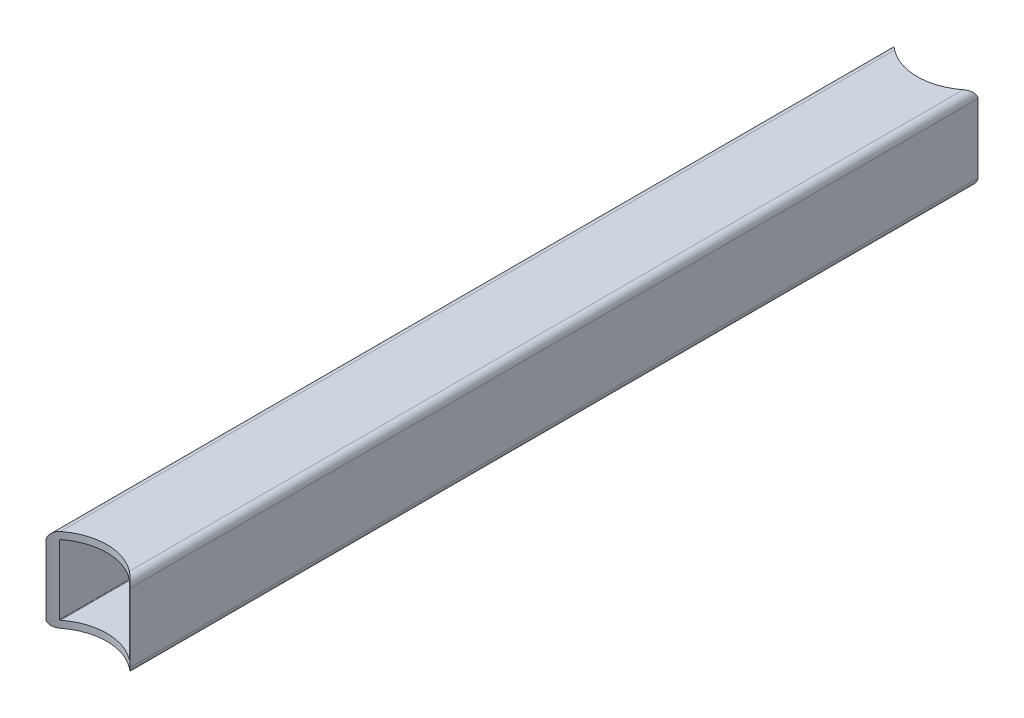
SolidWorks part; units mm, degrees
ref_plane "前视基准面" through (0, 0, 0) normal (0, 0, 1) x (1, 0, 0)
ref_plane "上视基准面" through (0, 0, 0) normal (0, 1, 0) x (1, 0, 0)
ref_plane "右视基准面" through (0, 0, 0) normal (1, 0, 0) x (0, 0, -1)
sketch "草图2" plane through (0, 0, 0) normal (0, 0, 1) x (1, 0, 0)
  line L1 (-12.3, 15) -> (12.3, 15)
  line L2 (-15, 12.3) -> (-15, -12.3)
  line L3 (-12.3, -15) -> (12.3, -15)
  line L4 (15, 12.3) -> (15, -12.3)
  line L5 (0, -15) -> (0, 15) construction
  line L6 (-15, 0) -> (15, 0) construction
  arc A0 (-15, -12.3) -> (-12.3, -15) centre (-12.3, -12.3) ccw
  arc A1 (12.3, -15) -> (15, -12.3) centre (12.3, -12.3) ccw
  arc A2 (12.3, 15) -> (15, 12.3) centre (12.3, 12.3) cw
  arc A3 (-12.3, 15) -> (-15, 12.3) centre (-12.3, 12.3) ccw
  point P0 (0, 0)
  point P6 (-15, -15)
  point P12 (15, -15)
  dimension "D2" = 2.7
  dimension "D1" = 30
extrude "拉伸-薄壁1" add sketch "草图2" along normal mid plane 330 thin
sketch "草图3" plane through (0, 0, 0) normal (0, 1, 0) x (1, 0, 0)
  line L0 (0, 0) -> (92.94, 0) construction
  circle A0 centre (0, -165) radius 20
  circle A1 centre (0, 165) radius 20
  dimension "D1" = 40
  dimension "D2" = 330
extrude "切除-拉伸1" cut sketch "草图3" against normal mid plane 50
